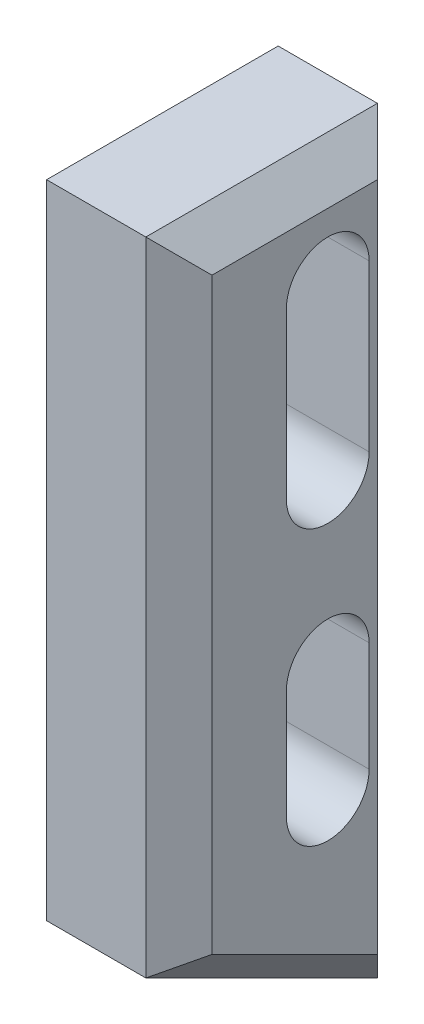
SolidWorks part; units mm, degrees
material "Q235-A"
ref_plane "Front Plane" through (0, 0, 0) normal (0, 0, 1) x (1, 0, 0)
ref_plane "Top Plane" through (0, 0, 0) normal (0, 1, 0) x (1, 0, 0)
ref_plane "Right Plane" through (0, 0, 0) normal (1, 0, 0) x (0, 0, -1)
sketch "Sketch1" plane through (0, 0, 0) normal (1, 0, 0) x (0, 0, -1)
  line L0 (0, 0) -> (70, -35)
  line L1 (70, -35) -> (70, 194)
  line L2 (70, 194) -> (0, 194)
  line L3 (0, 194) -> (0, 0)
  line L4 (45, 114) -> (45, 164) construction
  line L5 (32.5, 114) -> (32.5, 164)
  line L6 (57.5, 114) -> (57.5, 164)
  line L7 (45, 30.9103) -> (45, 64) construction
  line L8 (32.5, 30.9103) -> (32.5, 64)
  line L9 (57.5, 30.9103) -> (57.5, 64)
  arc A0 (32.5, 114) -> (57.5, 114) centre (45, 114) ccw
  arc A1 (57.5, 164) -> (32.5, 164) centre (45, 164) ccw
  arc A2 (32.5, 30.9103) -> (57.5, 30.9103) centre (45, 30.9103) ccw
  arc A3 (57.5, 64) -> (32.5, 64) centre (45, 64) ccw
  point P8 (45, 139)
  point P13 (45, 47.4552)
  dimension "D4" = 12.5
  dimension "D5" = 30
  dimension "D6" = 50
  dimension "D7" = 50
  dimension "D8" = 25
  dimension "D1" = 70
  dimension "D2" = 229
  dimension "D3" = 35
extrude "Boss-Extrude1" add sketch "Sketch1" along normal mid plane 40
chamfer "Chamfer1" distance 10 angle 45 4 edges at (20, -17.5, -35) (20, 97, 0) (20, 79.5, -70) (20, 194, -35)
